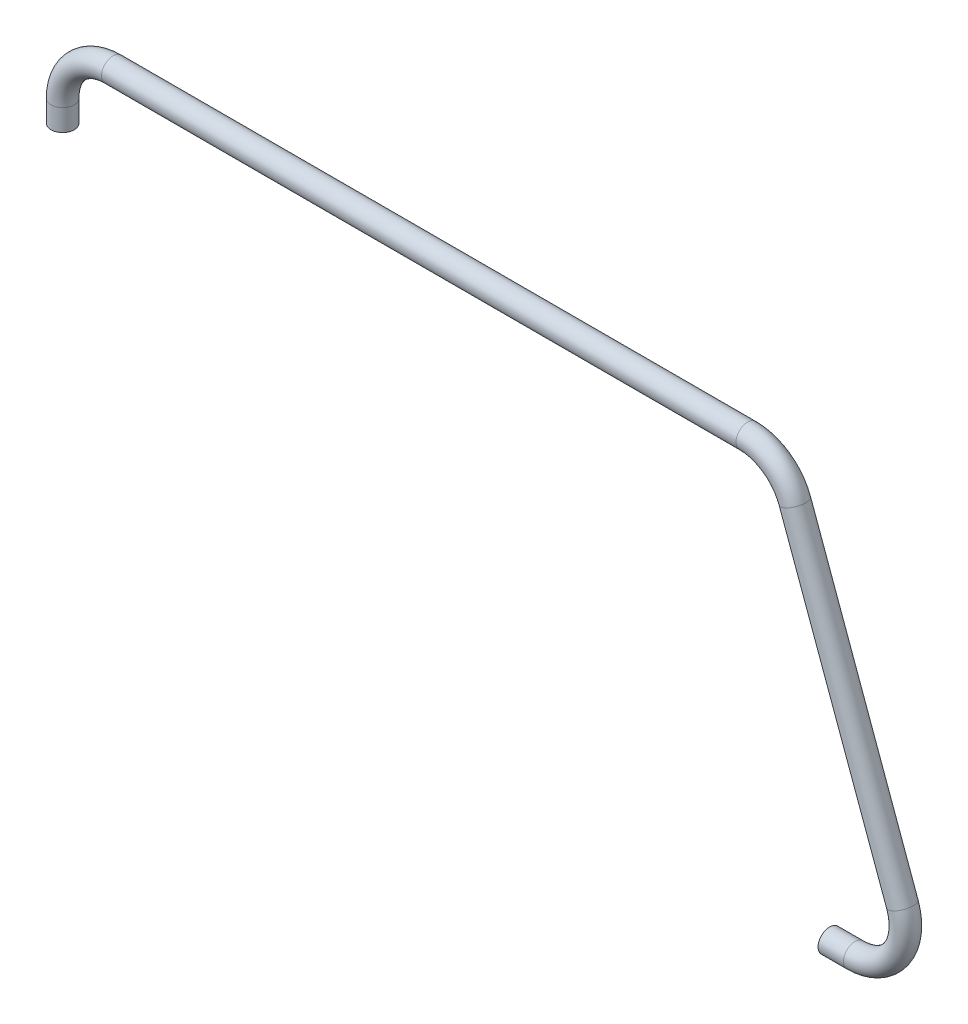
SolidWorks part; units mm, degrees
material "Q235B"
ref_plane "Front Plane" through (0, 0, 0) normal (0, 0, 1) x (1, 0, 0)
ref_plane "Top Plane" through (0, 0, 0) normal (0, 1, 0) x (1, 0, 0)
ref_plane "Right Plane" through (0, 0, 0) normal (1, 0, 0) x (0, 0, -1)
sketch "Sketch1" plane through (0, 0, 0) normal (0, 0, 1) x (1, 0, 0)
  line L0 (0, 0) -> (0, 30)
  line L1 (70, 100) -> (950.9855, 100)
  line L2 (1016.764, 53.9414) -> (1165.9918, -356.0586)
  line L3 (1100.2133, -450) -> (1065, -450)
  arc A0 (1165.9918, -356.0586) -> (1100.2133, -450) centre (1100.2133, -380) cw
  arc A1 (950.9855, 100) -> (1016.764, 53.9414) centre (950.9855, 30) cw
  arc A2 (0, 30) -> (70, 100) centre (70, 30) cw
  point P10 (1000, 100)
  point P13 (0, 100)
  dimension "D6" = 70
  dimension "D1" = 100
  dimension "D2" = 1000
  dimension "D3" = 550
  dimension "D4" = 110
  dimension "D5" = 1065
sketch "Sketch2" plane through (0, 0, 0) normal (0, 1, 0) x (1, 0, 0)
  circle A0 centre (0, 0) radius 16
  circle A1 centre (0, 0) radius 13
  dimension "D1" = 32
  dimension "D2" = 3
sweep "Sweep1" add profiles "Sketch2" path "Sketch1"
